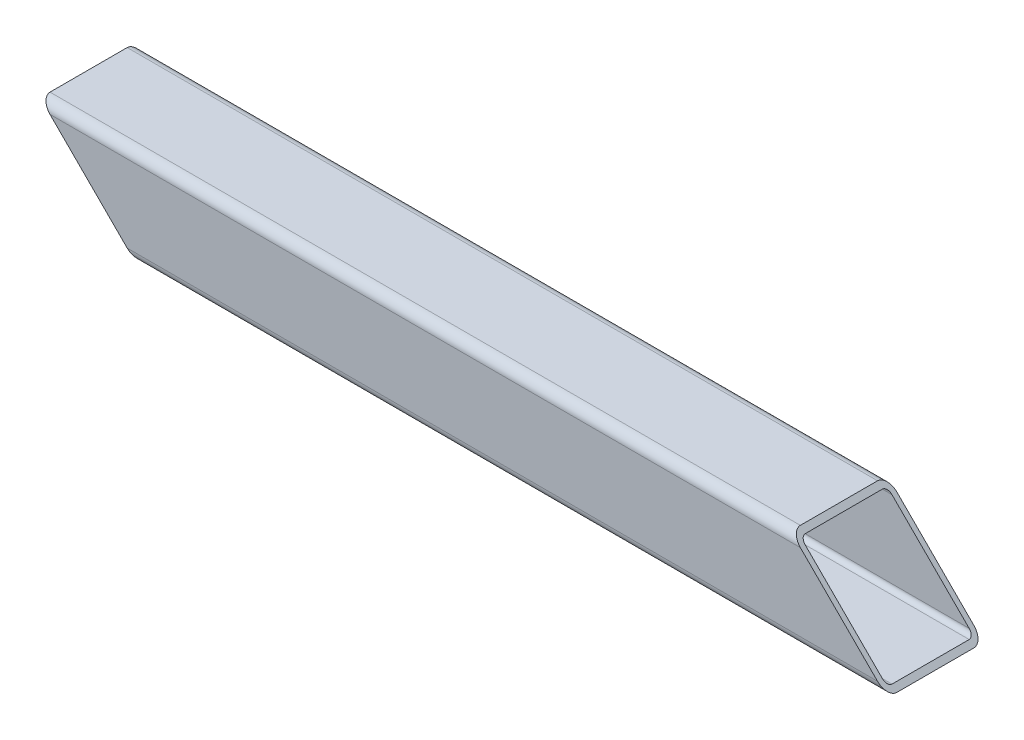
SolidWorks part; units mm, degrees
material "普通碳钢"
ref_plane "前视基准面" through (0, 0, 0) normal (0, 0, 1) x (1, 0, 0)
ref_plane "上视基准面" through (0, 0, 0) normal (0, 1, 0) x (1, 0, 0)
ref_plane "右视基准面" through (0, 0, 0) normal (1, 0, 0) x (0, 0, -1)
sketch3d "3D草图1"
  line L0 (0, 0, 0) -> (900, 0, 0)
  dimension "D1" = 900
other "方形管 100 X 100 X 5(1)"
ref_plane "基准面1" through (0, 0, 0) normal (1, 0, 0) x (0, 0, -1)
sketch "Sketch1" plane through (0, 0, 0) normal (1, 0, 0) x (0, 0, -1)
  line L0 (-40, -45) -> (40, -45)
  line L1 (-45, -40) -> (-45, 40)
  line L2 (40, 45) -> (-40, 45)
  line L3 (45, 40) -> (45, -40)
  line L4 (-40, -50) -> (40, -50)
  line L5 (-50, -40) -> (-50, 40)
  line L6 (40, 50) -> (-40, 50)
  line L7 (50, 40) -> (50, -40)
  arc A0 (50, 40) -> (40, 50) centre (40, 40) ccw
  arc A1 (40, -50) -> (50, -40) centre (40, -40) ccw
  arc A2 (-50, -40) -> (-40, -50) centre (-40, -40) ccw
  arc A3 (-40, 50) -> (-50, 40) centre (-40, 40) ccw
  arc A4 (-40, 45) -> (-45, 40) centre (-40, 40) ccw
  arc A5 (45, 40) -> (40, 45) centre (40, 40) ccw
  arc A6 (40, -45) -> (45, -40) centre (40, -40) ccw
  arc A7 (-45, -40) -> (-40, -45) centre (-40, -40) ccw
  point P0 (-50, 0)
  point P1 (50, 0)
  point P2 (0, 50)
  point P3 (0, -50)
  point P4 (0, 0)
  point P5 (-50, -50)
  point P6 (50, -50)
  point P7 (50, 50)
  point P8 (-50, 50)
  point P33 (0, 0)
  dimension "D1" = 10
  dimension "Thickness" = 5
  dimension "V_leg" = 100
sketch "草图2" plane through (0, 0, 50) normal (0, 0, 1) x (1, 0, 0)
  line L0 (0, 50) -> (100, -50)
  line L1 (900, -50) -> (0, -50) construction
  line L2 (100, -50) -> (0, -50)
  line L3 (0, -50) -> (0, 50)
  line L4 (913.7892, -85.9717) -> (913.7892, 50)
  line L5 (900, 50) -> (0, 50) construction
  line L6 (913.7892, 50) -> (777.8175, 50)
  line L7 (777.8175, 50) -> (913.7892, -85.9717)
  dimension "D1" = 45
  dimension "D2" = 550
extrude "切除-拉伸1" cut sketch "草图2" against normal blind 100
